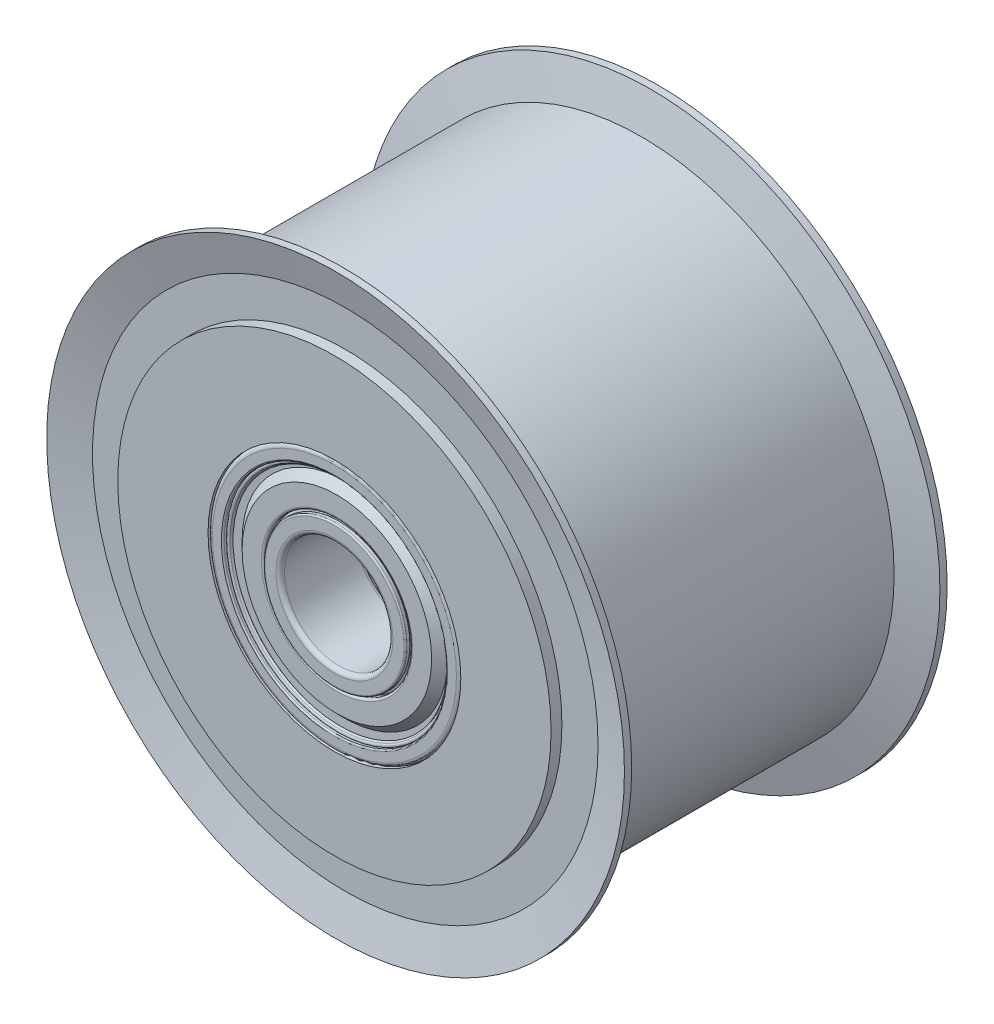
SolidWorks part; units mm, degrees
ref_plane "前视基准面" through (0, 0, 0) normal (0, 0, 1) x (1, 0, 0)
ref_plane "上视基准面" through (0, 0, 0) normal (0, 1, 0) x (1, 0, 0)
ref_plane "右视基准面" through (0, 0, 0) normal (1, 0, 0) x (0, 0, -1)
sketch "草图1" plane through (0, 0, 0) normal (1, 0, 0) x (0, 0, -1)
  line L0 (0, 17.5) -> (11, 17.5)
  line L1 (11, 17.5) -> (11, 12.75)
  line L2 (11, 12.75) -> (34, 12.75)
  line L3 (34, 12.75) -> (34, 17.5)
  line L4 (34, 17.5) -> (45, 17.5)
  line L5 (45, 17.5) -> (45, 30)
  line L6 (45, 30) -> (43.5, 30)
  line L7 (43.5, 30) -> (43.5, 35)
  line L8 (43.5, 35) -> (44.8397, 40)
  line L9 (44.8397, 40) -> (43.8397, 40)
  line L10 (43.8397, 40) -> (42.5, 35)
  line L11 (42.5, 35) -> (2.5, 35)
  line L12 (2.5, 35) -> (1.1603, 40)
  line L13 (1.1603, 40) -> (0.1603, 40)
  line L14 (0.1603, 40) -> (1.5, 35)
  line L15 (1.5, 35) -> (1.5, 30)
  line L16 (1.5, 30) -> (0, 30)
  line L17 (0, 30) -> (0, 17.5)
  line L18 (45, 0) -> (0, 0) construction
revolve "旋转1" add sketch "草图1" angle 360 about L18
ref_plane "基准面1" through (0, 0, -11) normal (0, 0, 1) x (1, 0, 0)
ref_plane "基准面2" through (0, 0, -11) normal (0, 0, 1) x (1, 0, 0)
ref_plane "基准面3" through (0, 0, -11) normal (0, 0, 1) x (1, 0, 0)
ref_plane "基准面4" through (0, 0, -11) normal (0, 0, 1) x (1, 0, 0)
ref_plane "基准面5" through (0, 0, -11) normal (0, 0, 1) x (1, 0, 0)
ref_plane "基准面6" through (0, 0, -11) normal (0, 0, 1) x (1, 0, 0)
sketch "草图2" plane through (0, 0, 0) normal (1, 0, 0) x (0, 0, -1)
  line L0 (0.2, 15.45) -> (0.5, 15.45)
  line L1 (0.5734, 15.0324) -> (0.819, 14.86)
  line L2 (0.819, 14.86) -> (0.991, 15.105)
  line L3 (0.991, 15.105) -> (0.746, 15.278)
  line L4 (0.746, 15.278) -> (1.0284, 15.6806)
  line L5 (1.392, 15.5731) -> (1.442, 14.224)
  line L6 (1.442, 14.224) -> (0.342, 13.124)
  line L7 (0.342, 13.124) -> (0.342, 10.45)
  line L8 (0.642, 10.15) -> (1.162, 10.15)
  line L9 (1.162, 10.15) -> (1.162, 10.45)
  line L10 (1.162, 10.45) -> (0.642, 10.45)
  line L11 (0.642, 10.45) -> (0.642, 13)
  line L12 (0.642, 13) -> (1.742, 14.1)
  line L13 (1.742, 14.1) -> (1.742, 14.45)
  line L14 (1.742, 14.45) -> (2.994, 14.45)
  line L15 (2.994, 10.55) -> (1.9451, 10.55)
  line L16 (1.7572, 10.4184) -> (1.4342, 9.5316)
  line L17 (1.2463, 9.4) -> (1.0708, 9.4)
  line L18 (0.9176, 9.4714) -> (0.6, 9.85)
  line L19 (0.6, 9.85) -> (0.2, 9.85)
  line L20 (0, 9.65) -> (0, 8.1)
  line L21 (0.6, 7.5) -> (10.4, 7.5)
  line L22 (11, 8.1) -> (11, 9.65)
  line L23 (10.8, 9.85) -> (10.4, 9.85)
  line L24 (10.4, 9.85) -> (10.0824, 9.4714)
  line L25 (9.9292, 9.4) -> (9.7537, 9.4)
  line L26 (9.5658, 9.5316) -> (9.2428, 10.4184)
  line L27 (9.0549, 10.55) -> (8.006, 10.55)
  line L28 (8.006, 14.45) -> (9.258, 14.45)
  line L29 (9.258, 14.45) -> (9.258, 14.1)
  line L30 (9.258, 14.1) -> (10.358, 13)
  line L31 (10.358, 13) -> (10.358, 10.45)
  line L32 (10.358, 10.45) -> (9.838, 10.45)
  line L33 (9.838, 10.45) -> (9.838, 10.15)
  line L34 (9.838, 10.15) -> (10.358, 10.15)
  line L35 (10.658, 10.45) -> (10.658, 13.124)
  line L36 (10.658, 13.124) -> (9.558, 14.224)
  line L37 (9.558, 14.224) -> (9.608, 15.5731)
  line L38 (9.9716, 15.6806) -> (10.254, 15.278)
  line L39 (10.254, 15.278) -> (10.009, 15.105)
  line L40 (10.009, 15.105) -> (10.181, 14.86)
  line L41 (10.181, 14.86) -> (10.4266, 15.0324)
  line L42 (10.5, 15.45) -> (10.8, 15.45)
  line L43 (11, 15.65) -> (11, 16.9)
  line L44 (10.4, 17.5) -> (0.6, 17.5)
  line L45 (0, 16.9) -> (0, 15.65)
  line L46 (50, 0) -> (-50, 0) construction
  arc A0 (0, 15.65) -> (0.2, 15.45) centre (0.2, 15.65) ccw
  arc A1 (0.5, 15.45) -> (0.5734, 15.0324) centre (0.7458, 15.278) ccw
  arc A2 (1.0284, 15.6806) -> (1.392, 15.5731) centre (1.1921, 15.5657) cw
  arc A3 (0.342, 10.45) -> (0.642, 10.15) centre (0.642, 10.45) ccw
  arc A4 (2.994, 14.45) -> (2.994, 10.55) centre (5.4996, 12.5) ccw
  arc A5 (1.9451, 10.55) -> (1.7572, 10.4184) centre (1.9451, 10.35) ccw
  arc A6 (1.4342, 9.5316) -> (1.2463, 9.4) centre (1.2463, 9.6) cw
  arc A7 (1.0708, 9.4) -> (0.9176, 9.4714) centre (1.0708, 9.6) cw
  arc A8 (0.2, 9.85) -> (0, 9.65) centre (0.2, 9.65) ccw
  arc A9 (0, 8.1) -> (0.6, 7.5) centre (0.6, 8.1) ccw
  arc A10 (10.4, 7.5) -> (11, 8.1) centre (10.4, 8.1) ccw
  arc A11 (11, 9.65) -> (10.8, 9.85) centre (10.8, 9.65) ccw
  arc A12 (10.0824, 9.4714) -> (9.9292, 9.4) centre (9.9292, 9.6) cw
  arc A13 (9.7537, 9.4) -> (9.5658, 9.5316) centre (9.7537, 9.6) cw
  arc A14 (9.2428, 10.4184) -> (9.0549, 10.55) centre (9.0549, 10.35) ccw
  arc A15 (8.006, 10.55) -> (8.006, 14.45) centre (5.5004, 12.5) ccw
  arc A16 (10.358, 10.15) -> (10.658, 10.45) centre (10.358, 10.45) ccw
  arc A17 (9.608, 15.5731) -> (9.9716, 15.6806) centre (9.8079, 15.5657) cw
  arc A18 (10.4266, 15.0324) -> (10.5, 15.45) centre (10.2542, 15.278) ccw
  arc A19 (10.8, 15.45) -> (11, 15.65) centre (10.8, 15.65) ccw
  arc A20 (11, 16.9) -> (10.4, 17.5) centre (10.4, 16.9) ccw
  arc A21 (0.6, 17.5) -> (0, 16.9) centre (0.6, 16.9) ccw
revolve "旋转2" add sketch "草图2" angle 360 about L46
sketch "草图3" plane through (0, 0, 0) normal (1, 0, 0) x (0, 0, -1)
  line L0 (34.2, 15.45) -> (34.5, 15.45)
  line L1 (34.5734, 15.0324) -> (34.819, 14.86)
  line L2 (34.819, 14.86) -> (34.991, 15.105)
  line L3 (34.991, 15.105) -> (34.746, 15.278)
  line L4 (34.746, 15.278) -> (35.0284, 15.6806)
  line L5 (35.392, 15.5731) -> (35.442, 14.224)
  line L6 (35.442, 14.224) -> (34.342, 13.124)
  line L7 (34.342, 13.124) -> (34.342, 10.45)
  line L8 (34.642, 10.15) -> (35.162, 10.15)
  line L9 (35.162, 10.15) -> (35.162, 10.45)
  line L10 (35.162, 10.45) -> (34.642, 10.45)
  line L11 (34.642, 10.45) -> (34.642, 13)
  line L12 (34.642, 13) -> (35.742, 14.1)
  line L13 (35.742, 14.1) -> (35.742, 14.45)
  line L14 (35.742, 14.45) -> (36.994, 14.45)
  line L15 (36.994, 10.55) -> (35.9451, 10.55)
  line L16 (35.7572, 10.4184) -> (35.4342, 9.5316)
  line L17 (35.2463, 9.4) -> (35.0708, 9.4)
  line L18 (34.9176, 9.4714) -> (34.6, 9.85)
  line L19 (34.6, 9.85) -> (34.2, 9.85)
  line L20 (34, 9.65) -> (34, 8.1)
  line L21 (34.6, 7.5) -> (44.4, 7.5)
  line L22 (45, 8.1) -> (45, 9.65)
  line L23 (44.8, 9.85) -> (44.4, 9.85)
  line L24 (44.4, 9.85) -> (44.0824, 9.4714)
  line L25 (43.9292, 9.4) -> (43.7537, 9.4)
  line L26 (43.5658, 9.5316) -> (43.2428, 10.4184)
  line L27 (43.0549, 10.55) -> (42.006, 10.55)
  line L28 (42.006, 14.45) -> (43.258, 14.45)
  line L29 (43.258, 14.45) -> (43.258, 14.1)
  line L30 (43.258, 14.1) -> (44.358, 13)
  line L31 (44.358, 13) -> (44.358, 10.45)
  line L32 (44.358, 10.45) -> (43.838, 10.45)
  line L33 (43.838, 10.45) -> (43.838, 10.15)
  line L34 (43.838, 10.15) -> (44.358, 10.15)
  line L35 (44.658, 10.45) -> (44.658, 13.124)
  line L36 (44.658, 13.124) -> (43.558, 14.224)
  line L37 (43.558, 14.224) -> (43.608, 15.5731)
  line L38 (43.9716, 15.6806) -> (44.254, 15.278)
  line L39 (44.254, 15.278) -> (44.009, 15.105)
  line L40 (44.009, 15.105) -> (44.181, 14.86)
  line L41 (44.181, 14.86) -> (44.4266, 15.0324)
  line L42 (44.5, 15.45) -> (44.8, 15.45)
  line L43 (45, 15.65) -> (45, 16.9)
  line L44 (44.4, 17.5) -> (34.6, 17.5)
  line L45 (34, 16.9) -> (34, 15.65)
  line L46 (50, 0) -> (-50, 0) construction
  arc A0 (34, 15.65) -> (34.2, 15.45) centre (34.2, 15.65) ccw
  arc A1 (34.5, 15.45) -> (34.5734, 15.0324) centre (34.7458, 15.278) ccw
  arc A2 (35.0284, 15.6806) -> (35.392, 15.5731) centre (35.1921, 15.5657) cw
  arc A3 (34.342, 10.45) -> (34.642, 10.15) centre (34.642, 10.45) ccw
  arc A4 (36.994, 14.45) -> (36.994, 10.55) centre (39.4996, 12.5) ccw
  arc A5 (35.9451, 10.55) -> (35.7572, 10.4184) centre (35.9451, 10.35) ccw
  arc A6 (35.4342, 9.5316) -> (35.2463, 9.4) centre (35.2463, 9.6) cw
  arc A7 (35.0708, 9.4) -> (34.9176, 9.4714) centre (35.0708, 9.6) cw
  arc A8 (34.2, 9.85) -> (34, 9.65) centre (34.2, 9.65) ccw
  arc A9 (34, 8.1) -> (34.6, 7.5) centre (34.6, 8.1) ccw
  arc A10 (44.4, 7.5) -> (45, 8.1) centre (44.4, 8.1) ccw
  arc A11 (45, 9.65) -> (44.8, 9.85) centre (44.8, 9.65) ccw
  arc A12 (44.0824, 9.4714) -> (43.9292, 9.4) centre (43.9292, 9.6) cw
  arc A13 (43.7537, 9.4) -> (43.5658, 9.5316) centre (43.7537, 9.6) cw
  arc A14 (43.2428, 10.4184) -> (43.0549, 10.55) centre (43.0549, 10.35) ccw
  arc A15 (42.006, 10.55) -> (42.006, 14.45) centre (39.5004, 12.5) ccw
  arc A16 (44.358, 10.15) -> (44.658, 10.45) centre (44.358, 10.45) ccw
  arc A17 (43.608, 15.5731) -> (43.9716, 15.6806) centre (43.8079, 15.5657) cw
  arc A18 (44.4266, 15.0324) -> (44.5, 15.45) centre (44.2542, 15.278) ccw
  arc A19 (44.8, 15.45) -> (45, 15.65) centre (44.8, 15.65) ccw
  arc A20 (45, 16.9) -> (44.4, 17.5) centre (44.4, 16.9) ccw
  arc A21 (34.6, 17.5) -> (34, 16.9) centre (34.6, 16.9) ccw
revolve "旋转3" add sketch "草图3" angle 360 about L46
other "冻结***"
